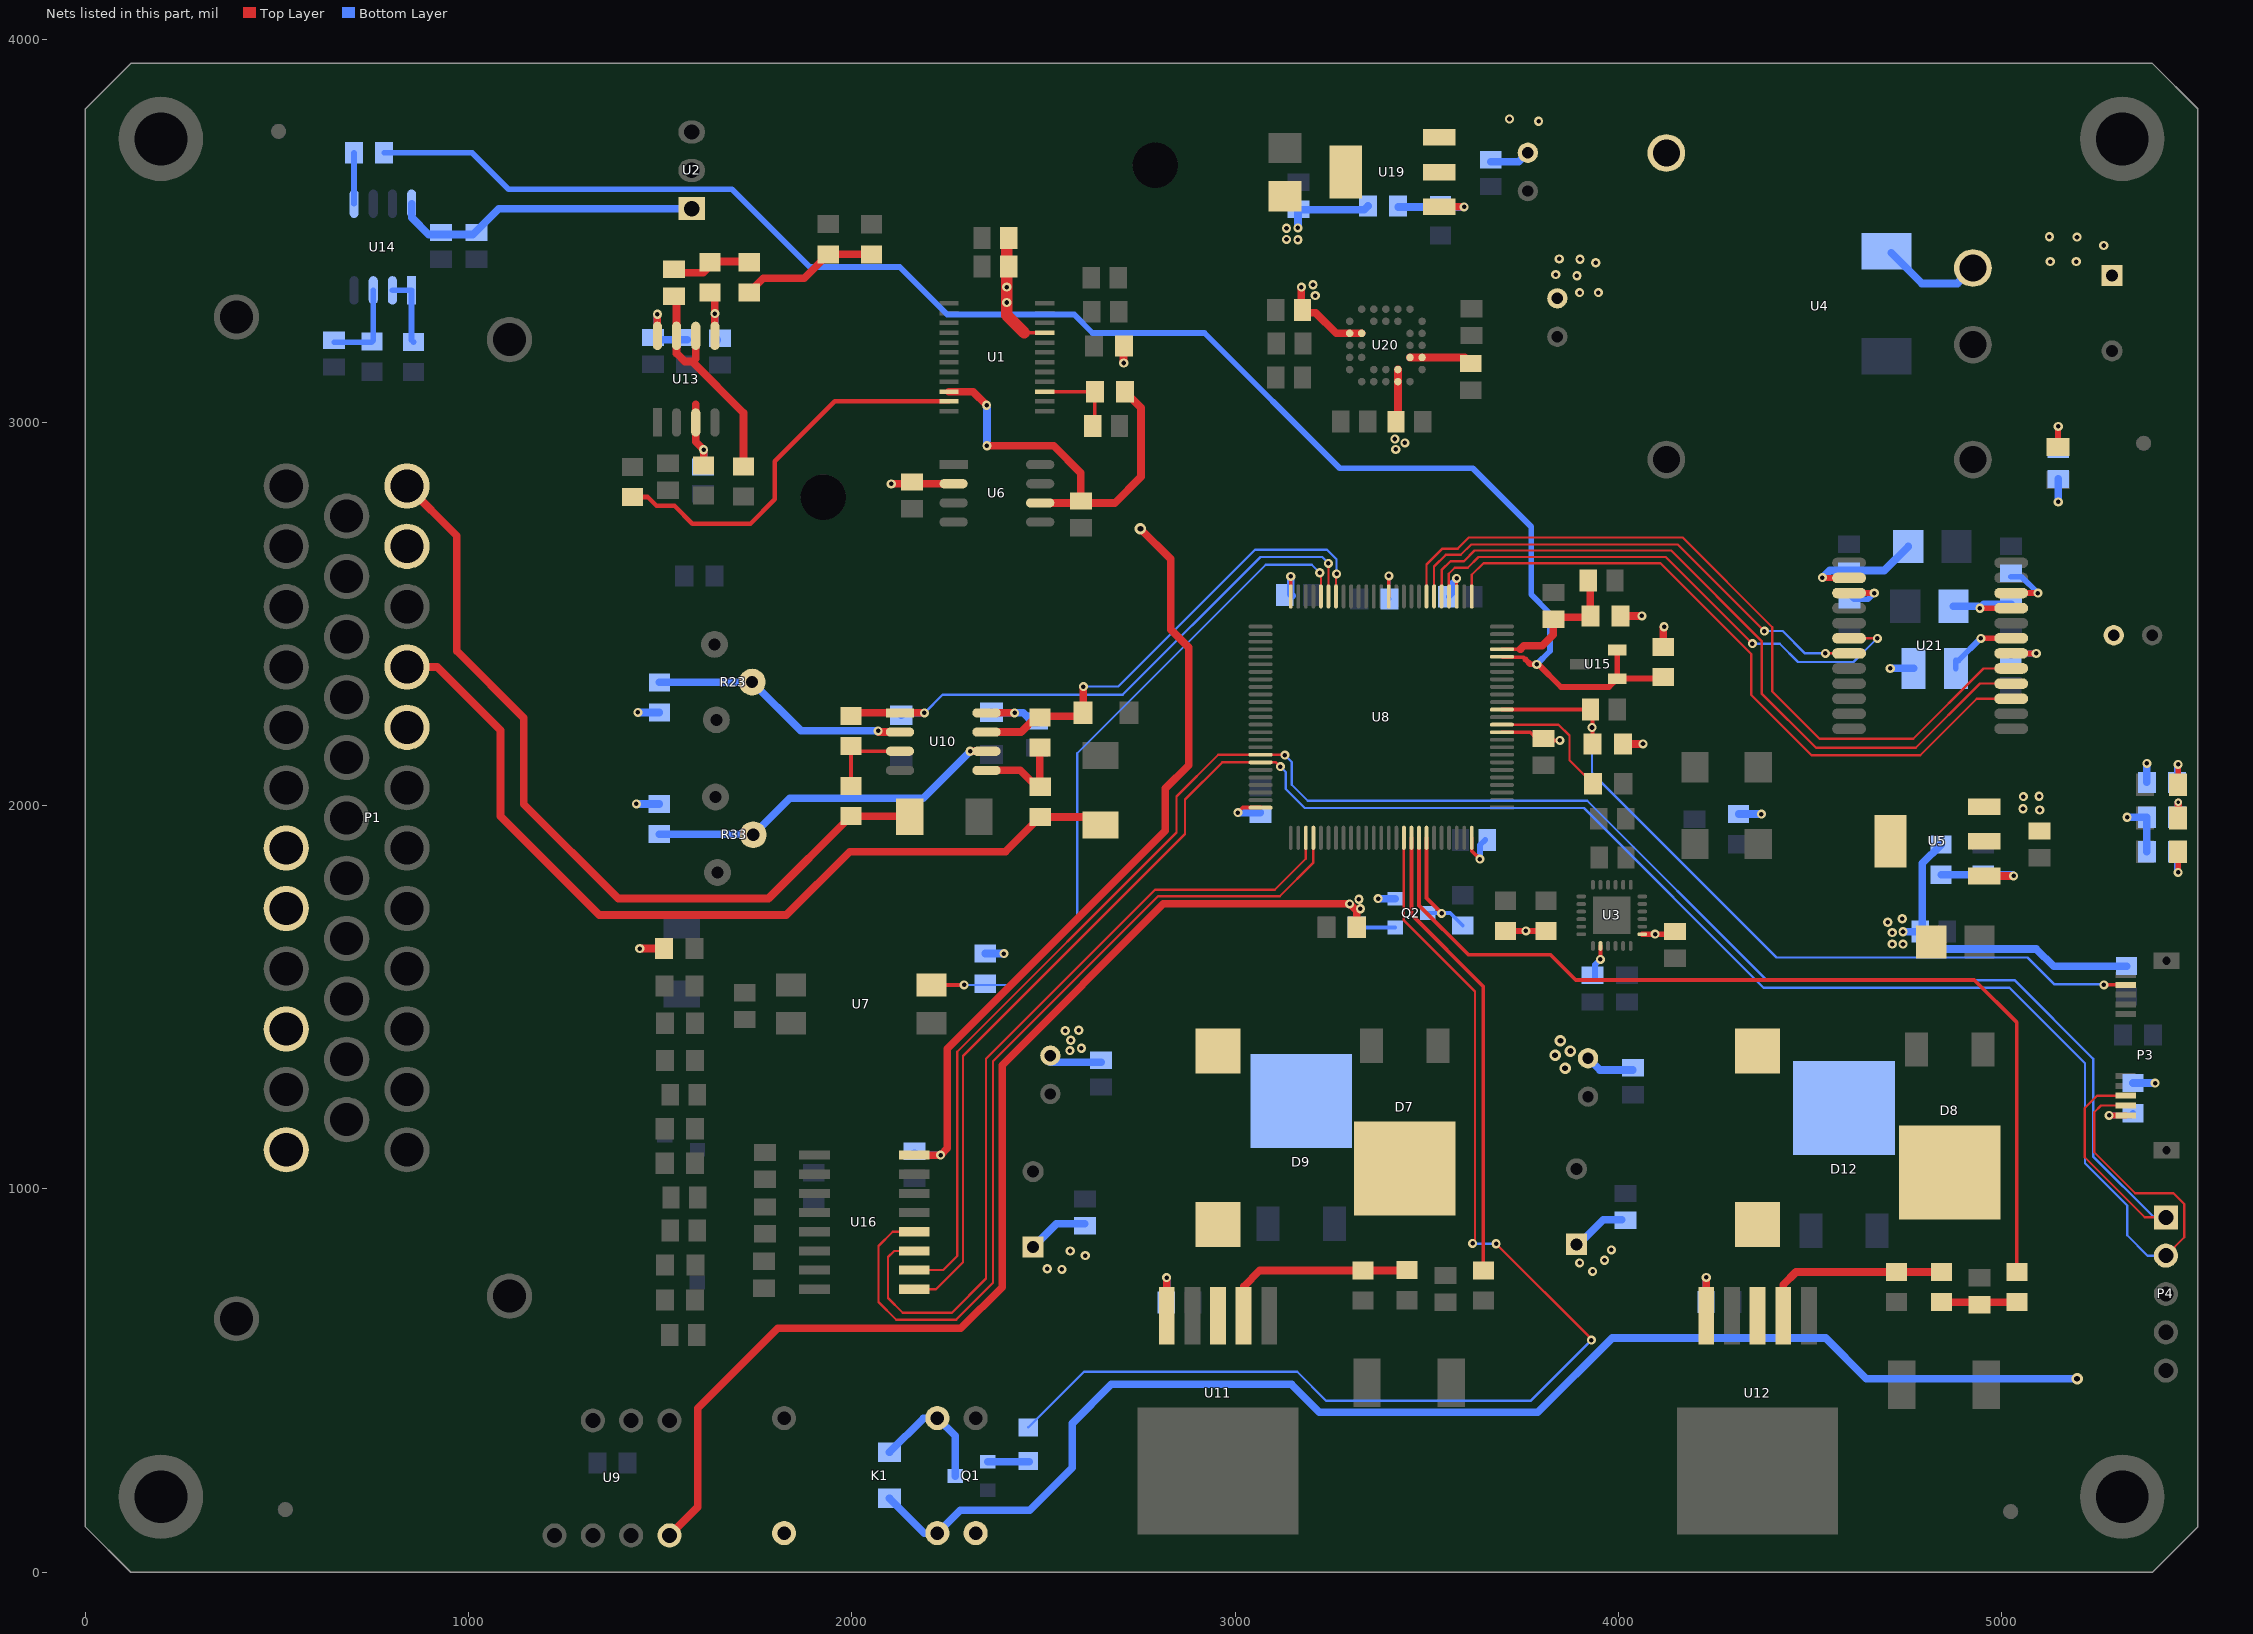
[diagram p0: the nets of this part, all layers, seen from the top]
# Altium PCB MISC82155.PcbDoc (part 4 of 5)
Units mil, origin at the board's own origin, x right, y up, seen from the top; angles counter-clockwise.
Board outline 5511.81 x 3937.01 mil, 4 copper layers (Top Layer, GND, POWER, Bottom Layer); 191 components, 134 nets, 709 pads, 440 vias.

## Via types
v1: diameter 24, hole 12, Top Layer to Bottom Layer, 278 vias
v2: diameter 23.62, hole 11.81, Top Layer to Bottom Layer, 144 vias
v3: diameter 30, hole 15, Top Layer to Bottom Layer, 17 vias
v4: diameter 20, hole 10, Top Layer to Bottom Layer, 1 vias

## Nets (pads, with @x,y where several pads share a name; then routed paths per layer and width w, separated by ;. In a path a pad name is that pad's centre, name@x,y a point inside that pad or via, vN(x,y) a via of type N, cw(c..) or ccw(c..) an arc to the next point about the centre after c; other vN are vias at no path point) (continued)
NetC60_2: C60.2 U20.C1 U20.C2 | length 165.2
  Top Layer w20: U20.C2@3456.4,3169.85 U20.C1@3487.89,3169.85 3599.15,3169.85 C60.2@3615,3154
NetC65_1: C65.1 U21.15 | length 143
  Top Layer w15: U21.15@4602.17,2555.09 v2(4667.91,2555.09)
  Bottom Layer w15: C65.1@4602.66,2551.93 4615.59,2539 4651.83,2539 v2(4667.91,2555.09)
NetC66_1: C66.1 U21.10 | length 157.5
  Top Layer w15: U21.10@5025.4,2555.09 v2(5094.91,2555.09)
  Bottom Layer w15: C66.1@5024.66,2597.88 5052.12,2597.88 v2(5094.91,2555.09)
NetC67_1: C67.1 U21.6 | length 132.9
  Top Layer w15: U21.6@5025.4,2397.61 v2(5090.61,2397.61)
  Bottom Layer w15: C67.1@5025.66,2390.93 5032.33,2397.61 v2(5090.61,2397.61)
NetC69_1: C69.1 R31.2 R37.2 | length 197
  Top Layer w20: R31.2@4843,704.63 R37.2@5040,704.63
NetC71_1: C71.1 R43.1 U13.6 U13.7 | length 601.4
  Top Layer w20: C71.1@1543.41,3331.81 1542.41,3330.81 U13.7@1542.41,3226.34 1542.41,3180.34 1563.41,3159.34 1583,3159.34 1717,3025.34 R43.1@1717,2893.31 ; 1592.41,3166.34 1592.41,3178.34 U13.6@1592.41,3226.34 ; R43.1@1709.41,2885.71 R43.1@1717,2893.31 ; R43.1@1717,2885.37 R43.1@1717,2893.31
NetC71_2: C71.2 R47.2 R48.1 | length 212.4
  Top Layer w20: C71.2@1551.04,3398.5 1543.41,3390.87 1612.5,3390.87 1642,3420.37 1730,3420.37 R47.2@1732,3418.37
NetC72_1: C72.1 R46.2 U13.3 | length 218.8
  Top Layer w20: 1592.41,3047.34 U13.3@1592.41,3000.34 1592.41,2949.59 v2(1613,2929) R46.2@1613,2888.37
  Bottom Layer w20: C72.1@1611,2878.53 1613,2880.53 v2(1613,2929)
NetC73_1: C73.1 R48.2 U13.5 | length 186.7
  Top Layer w20: R48.2@1642,3341.63 1642,3284.41 v2(1642.41,3284) U13.5@1642.41,3226.34
  Bottom Layer w20: v2(1642.41,3284) 1642.41,3222.12 C73.1@1649,3215.53
NetC78_1: C78.1 R61.1 U14.3 | length 234.6
  Bottom Layer w15: C78.1@649,3209.53 746.16,3209.53 751,3214.37 U14.3@751,3345
NetD1_1: D1.1 R5.1 | length 109.2
  Top Layer w15: v2(5461,1826) D1.1@5461,1880
  Bottom Layer w15: R5.1@5458.06,1880 5458.06,1828.94 v2(5461,1826)
NetD2_1: D2.1 R7.1 | length 81.8
  Top Layer w19.68: D2.1@5461,1968 v4(5461,2009) v4@5461,2009.63
  Bottom Layer w19.68: R7.1@5458.06,1970 5461,1972.94 v4(5461,2009)
NetD3_1: D3.1 R10.1 | length 101.2
  Top Layer w15: D3.1@5461,2055 v2(5461,2108)
  Bottom Layer w15: R10.1@5458.06,2061 5458.06,2105.06 v2(5461,2108)
NetD5_1: D5.1 R3.1 | length 112.2
  Top Layer w15: D5.1@5147.41,2936.65 5147.41,2989.41 v2(5148,2990)
  Bottom Layer w15: R3.1@5148,2931.37 v2(5148,2990)
NetD7_2: D7.2 L5.1 U11.3
NetD8_2: D8.2 L6.1 U12.3
NetD13_1: D13.1 K1.5 Q1.3 | length 332.1
  Bottom Layer w20: D13.1@2098,313 2187,402 K1.5@2223,402 2269.5,355.5 Q1.3@2269.5,251
NetL4_2: L4.2 U21.7 | length 189.1
  Top Layer w15: v2(4946.02,2436.98) U21.7@5025.4,2436.98
  Bottom Layer w15: L4.2@4880.78,2358.41 4880.78,2378.78 4887.82,2378.78 v2(4946.02,2436.98)
NetP3_1: P3.1 R60.2 | length 107.4
  Top Layer w15.75: v2(5281,1192.29) P3.1@5324.16,1192.29
  Bottom Layer w15.75: v2(5281,1192.29) 5337.66,1192.29 R60.2@5343,1197.63
NetQ1_1: Q1.1 R50.2 | length 107.7
  Bottom Layer w20: Q1.1@2354.5,288.4 2461.6,288.4 R50.2@2462,288
NetQ2_1: Q2.1 R34.1 | length 95.7
  Bottom Layer w10: R34.1@3322.03,1682.6 Q2.1@3417.65,1682.6
NetQ2_3: Q2.3 R28.2 U8.94 | length 317.5
  Top Layer w9.84: U8.94@3499.52,1916.38 3499.52,1759.48 v2@3539,1720
  Bottom Layer w9.84: Q2.3@3502.65,1720 3561.63,1720 R28.2@3594,1687.63
  other v2: 3539,1719
NetR2_1: R2.1 R47.1 R49.1 | length 360.3
  Top Layer w20: R47.1@1732,3339.63 1768.95,3376.58 1876.02,3376.58 1934.44,3435 R2.1@1938.41,3438.97 2050.66,3438.97 R49.1@2051,3438.63
NetR14_1: R14.1 R16.2 U11.2 | length 520.4
  Top Layer w20: U11.2@3022.34,669.34 3022.34,745.27 3064.44,787.37 R16.2@3334,787.37 3448,787.37 R14.1@3449,788.37
NetR15_2: R15.2 R19.1 U10.3 | length 237.9
  Top Layer w10: R19.1@1997.41,2051.71 R15.2@1997.41,2155.97 2011.04,2142.34 U10.3@2125.41,2142.34
NetR17_1: R17.1 R21.2 U19.1 | length 237.6
  Top Layer w20: U19.1@3532.33,3562.9 v2(3597.9,3562.9)
  Bottom Layer w20: R17.1@3426,3562.63 3597.63,3562.63 v2(3597.9,3562.9)
NetR22_1: R22.1 R23.2 U10.2 | length 680.7
  Top Layer w20: R23.2@1739.2,2322.14 R23.2@1739.83,2322.77 ; v1@2069.41,2192.34 U10.2@2125.41,2192.34
  Bottom Layer w20: R22.1@1497.62,2322.14 1739.2,2322.14 R23.2@1739.83,2322.77 1867.26,2195.34 v1(2068.41,2195.34)
NetR25_2: R25.2 R29.1 U10.5 | length 241.1
  Top Layer w20: U10.5@2351.41,2092.34 2439.66,2092.34 2469.66,2062.34 R29.1@2478.79,2062.34 ; R29.1@2490.41,2050.72 R25.2@2490.41,2151.97
NetR26_2: R26.2 R31.1 U12.2 | length 507.1
  Top Layer w20: U12.2@4430.34,669.34 4430.34,750 4463.71,783.37 R26.2@4726,783.37 R31.1@4843,783.37
NetR32_1: R32.1 R33.2 U10.6 | length 945
  Top Layer w20: v1(2308.41,2142.34) U10.6@2351.41,2142.34
  Bottom Layer w20: R32.1@1497.41,1925.97 1740.99,1925.97 R33.2@1742.62,1924.34 1838.28,2020 2186.07,2020 v1(2308.41,2142.34)
NetR35_1: R35.1 R38.2 U5.1 | length 268
  Top Layer w20: U5.1@4954.45,1816.79 v2(5031.79,1816.79)
  Bottom Layer w20: R35.1@4842.41,1819.97 R38.2@4952.41,1819.97 5028.61,1819.97 v2(5031.79,1816.79)
NetR39_2: R39.2 U1.11 | length 1045.1
  Top Layer w12: R39.2@1427,2805.63 1467.37,2805.63 1490,2783 1537,2783 1583.66,2736.34 1735.34,2736.34 1799,2800 1799,2898.93 1955.25,3055.18 U1.11@2253.41,3055.18
NetR54_1: R54.1 U14.1 U14.2 | length 186.7
  Bottom Layer w15: U14.2@801,3345 U14.1@851,3345 851,3215.37 R54.1@856,3210.37
NetR62_2: R62.2 U14.5 | length 132.6
  Bottom Layer w15: U14.5@701,3571 R62.2@701,3703.63
NRST: C17.2 P3.9 R24.1 U8.14 | length 2067.2
  Top Layer w9.84: U8.14@3696.37,2251.03 3932.56,2251.03 3932.88,2251.34 3932.88,2161.5 R24.1@3933.04,2161.34 ; v2(5267.16,1532.84) P3.9@5324.16,1532.84
  Bottom Layer w6: v1(3931.41,2204.34) 3931.41,2085.59 4413,1604 5068,1604 5138.16,1533.84 5266.16,1533.84 v2(5267.16,1532.84)
PB2_BOOT1: R20.2 U8.37 | length 115
  Top Layer w9.84: U8.37@3401.09,2546.3 v2(3401.09,2599.91)
  Bottom Layer w9.84: v2@3401,2600 v2(3401.09,2599.91) 3401.09,2541.03 R20.2@3402.78,2539.34
PD_IN: R9.2 U7.4 U8.46 | length 1812.4
  Top Layer w6: v2(3220.85,2608) 3223.93,2604.93 U8.46@3223.93,2546.3
  Top Layer w9.84: U7.4@2217.11,1522.71 U7.4@2207.48,1532.34 v2(2293,1532.34)
  Bottom Layer w6: v2(2293,1532.34) 2422.34,1532.34 2588,1698 2588,2137 3080,2629 3199.85,2629 v2(3220.85,2608)
  Bottom Layer w9.84: v2@2291.37,1530.71 v2(2293,1532.34)
REF1: C3.1 R1.1 U1.15 | length 219
  Top Layer w10: U1.15@2503.84,3080.34 R1.1@2634.04,3080.34 ; C3.1@2633.88,2991.34 R1.1@2633.88,3080.18
REF2V5: R18.2 R62.1 U8.21 U15.1 U15.2 | length 4336.2
  Top Layer w10: U8.21@3696.37,2388.82 3697.68,2387.51 3752.24,2387.51 3758.11,2381.64
  Top Layer w15: 3758.11,2381.64 3770.41,2369.34 3791,2369.34 3850.34,2310 3975.61,2310 U15.1@3997.21,2331.6 ; U15.2@3997.21,2406.4 U15.1@3997.21,2331.94 ; R18.2@4124.04,2331.94 U15.1@3997.55,2331.94 ; U15.1@3997.21,2331.6 U15.1@3997.55,2331.94 ; U15.1@3997.21,2331.6 U15.1@3997.21,2331.94 ; U15.1@3997.21,2331.94 U15.1@3997.55,2331.94
  Bottom Layer w15: R62.1@779.37,3704 1009,3704 1104,3609 1687,3609 1890,3406 2125,3406 2249,3282 2580,3282 2628,3234 2920,3234 3273,2881 3620,2881 3773,2728 3773,2551 3822,2502 3822,2404 v1(3787,2369)
REF2V5_1: C13.1 R1.2 U1.10 U6.6 | length 1101.4
  Top Layer w10: U6.6@2491.41,2790.34 U6.6@2491.88,2789.87
  Top Layer w20: U1.10@2253.41,3080.77 2315.97,3080.77 v1(2351.41,3045.34) ; v1(2352.41,2939.34) 2526.41,2939.34 2597.41,2868.34 C13.1@2597.41,2789.87 ; U6.6@2491.88,2789.87 C13.1@2597.41,2789.87 ; R1.2@2712.78,3080.34 2754.41,3038.71 2754.41,2858.34 2685.93,2789.87 C13.1@2597.41,2789.87
  Bottom Layer w20: v1(2352.41,2939.34) v1@2352.41,3044.34
RXD1: P3.2 P4.2 U8.69 U16.9 | length 5629.9
  Top Layer w6: U16.9@2191.41,738.34 U16.9@2162.41,738.34 2219.34,738.34 2290,809 2290,1347 2869,1926 2869,2016 2966.23,2113.23 U8.69@3066.45,2113.23 3106.77,2113.23 v2(3118,2102) ; P3.2@5324.16,1217.88 5259.88,1217.88 5242,1200 5242,1096 5349,989 5449,989 5477,961 5477,874 P4.2@5429,826
  Bottom Layer w6: v2(3118,2102) 3132,2088 3132,2044 3182,1994 3910.18,1994 4379.18,1525 5021,1525 5218,1328 5218,1067 5328,957 5328,879 5381,826 P4.2@5429,826
RXD2: U8.79 U16.12 | length 2305.5
  Top Layer w6: U16.12@2162.41,888.34 2106.41,888.34 2069.41,851.34 2069.41,705.34 2115.75,659 2272,659 2368,755 2368,1333 2799,1764 3116.24,1764 3204.24,1852 U8.79@3204.24,1916.38
SCC_CLK: U8.30 U21.4 | length 1939.2
  Top Layer w6: U8.30@3538.89,2546.3 3538.89,2614.89 3562,2638 3597,2638 3625,2666 4138,2666 4374,2430 4374,2293 4515.79,2151.21 4776.21,2151.21 4943.87,2318.87 U21.4@5025.4,2318.87
SCC_CS: U8.29 U21.18 | length 1409.2
  Top Layer w6: U8.29@3558.57,2546.3 3557.45,2547.43 3557.45,2605.45 3573,2621 3607,2621 3635,2649 4124,2649 v2(4350,2423) ; U21.18@4602.17,2436.98 v2(4675.98,2436.98)
  Bottom Layer w6: v2(4350,2423) 4421,2423 4469,2375 4614,2375 v2(4675.98,2436.98)
SCC_MISO: U8.32 U21.5 | length 2039.3
  Top Layer w6: U8.32@3499.52,2546.3 3499.52,2629.52 3541,2671 3581,2671 3610,2700 4168,2700 4402,2466 4402,2298 4524.97,2175.03 4769.79,2175.03 4953,2358.24 U21.5@5025.4,2358.24 U21.5@5034.66,2358.24
SCC_MOSI: U8.31 U21.19 | length 1371.2
  Top Layer w6: 3519.2,2579.55 U8.31@3519.2,2546.3 3519.2,2624.2 3550,2655 3589,2655 3616,2682 4155,2682 4364,2473 v2(4381,2456) ; v2(4540.61,2397.61) U21.19@4602.17,2397.61 U21.19@4566.86,2397.61
  Bottom Layer w6: v2(4381,2456) 4429,2456 4487.39,2397.61 v2(4540.61,2397.61)
SCC_RST: U8.26 U21.3 | length 1838.6
  Top Layer w6: U8.26@3617.63,2546.3 3617.63,2602.63 3648,2633 4110,2633 4347,2396 4347,2289 4504,2132 4788,2132 4935.5,2279.5 U21.3@5025.4,2279.5 U21.3@4994.75,2279.5
SEAT_PRESS: DW3.2 R15.1 U8.45 U10.1 | length 1581.1
  Top Layer w6: U8.45@3243.61,2546.3 v2(3243.61,2632.61)
  Top Layer w20: R15.1@1987,2242.34 U10.1@2125.41,2242.34 v2(2189.34,2242.34)
  Bottom Layer w6: v2(2189.34,2242.34) 2237,2290 2707,2290 3066,2649 3227.22,2649 v2(3243.61,2632.61)
  Bottom Layer w20: DW3.2@2129,2236 2135.34,2242.34 v2(2189.34,2242.34)
SEAT_SEN: D10.2 P1.1 R19.2 | length 2155.3
  Top Layer w20: P1.1@838.99,2834.48 969,2704.47 969,2404 1144,2229 1144,2004 1390,1758 1782.44,1758 R19.2@1997.41,1972.97 2149.23,1972.97 D10.2@2150.85,1971.34
SO_12V: C18.1 C19.1 C20.1 C33.1 C34.1 C38.1 K1.2 U11.5 U12.5 | length 637.2
  Top Layer w20: U11.5@2821.55,669.34 v2(2821.55,768.55) ; U12.5@4229.55,669.34 v2(4229.55,769.45)
  Bottom Layer w20: C18.1@2473,848.57 2533.9,909.47 C19.1@2608,909.47 ; v2(2821.55,768.55) 2821.55,707.92 C20.1@2825.47,704 ; C33.1@3891,855.57 3896.76,855.57 3961,919.81 C34.1@4009.41,919.81 ; v2(4229.55,769.45) 4229.55,709.92 C38.1@4234.47,705
  other v1: 3933,785 2548,790 2510,792 3899,807 3964,814 2609,826 2570,838 3982,841
SO_PW: R50.1 U8.91 | length 3179
  Top Layer w6: U8.91@3440.46,1916.38 3440.46,1700.54 3626,1515 3626,864 v2(3620,858) ; v2(3681,857) 3929.69,608.31 v2(3929.69,605.69)
  Bottom Layer w6: R50.1@2460,378 2461,378 2606,523 3162,523 3238,447 3771,447 v2(3929.69,605.69) ; v2@3621,857 v2(3681,857)
SOLENIOD_A: C21.1 C31.1 D9.2 L5.2 P1.35 | length 135.3
  Bottom Layer w20: C31.1@2515.41,1332.34 2517.22,1330.53 C21.1@2650,1330.53
  other v1: 2569,1361 2599,1367 2571,1388 2557,1413 2592,1414
SOLENIOD_B: C43.1 C68.1 D12.2 L6.2 P1.33 | length 129.6
  Bottom Layer w20: C68.1@3921,1341 3951.47,1310.53 C43.1@4038,1310.53
  other v3: 3861,1315 3835,1349 3875,1360 3849,1387
STWHEEL_SEN: D11.2 P1.4 R29.2 | length 2326.6
  Top Layer w20: P1.4@838.99,2362.04 917.96,2362.04 1083,2197 1083,1973 1341,1715 1829,1715 1994,1880 2400.67,1880 R29.2@2491.53,1970.86 D11.2@2660.41,1970.86
SUOFA_IN: DW4.2 R25.1 U8.44 U10.7 | length 1249.4
  Top Layer w6: U8.44@3263.3,2546.3 3263.3,2605.3 v2(3264.7,2605.3)
  Top Layer w20: U10.7@2351.41,2192.34 2441.34,2192.34 2479.71,2230.71 R25.1@2490.41,2230.71 ; R25.1@2489.41,2233.34 DW4.2@2598.04,2233.34 ; DW4.2@2603.41,2242.34 v2@2603.41,2311
  Bottom Layer w6: v2(2604,2311) 2695,2311 3052,2668 3240,2668 3264.7,2643.3 v2(3264.7,2605.3)
TXD1: P3.3 P4.1 U8.68 U16.10 | length 5433.6
  Top Layer w6: U16.10@2195.41,788.34 U16.10@2162.41,788.34 2238.34,788.34 2275,825 2275,1358 2847,1930 2847,2024 2955.92,2132.92 U8.68@3066.45,2132.92 3129.08,2132.92 v2(3130,2132) ; P3.3@5324.16,1243.47 5249.47,1243.47 5217,1211 5217,1083 5374,926 P4.1@5429,926
  Bottom Layer w6: v2(3130,2132) 3148,2114 3148,2054.57 3189.57,2013 3919,2013 4387,1545 5034,1545 5239,1340 5239,1085 5398,926 P4.1@5429,926
TXD2: U8.78 U16.11 | length 2169.1
  Top Layer w6: U16.11@2162.41,838.34 2110.41,838.34 2094.41,822.34 2094.41,715.34 2132.75,677 2261,677 2350,766 2350,1340 2791,1781 3103.56,1781 3184.56,1862 U8.78@3184.56,1916.38
VALVE_PWM1: R30.1 U8.92 | length 1223.8
  Top Layer w9.84: 3460.15,1876.08 3460.15,1884 ; U8.92@3460.15,1916.38 3460.15,1884 ; 3647.41,874.97 3647.41,884 ; R30.1@3648,787.37 3647.41,787.96 3647.41,884 ; 3460.15,1884 3460.15,1716 3647.41,1528.74 3647.41,884
VALVE_PWM2: R37.1 U8.93 | length 2513.9
  Top Layer w9.84: U8.93@3479.83,1916.38 3479.83,1740 3608.83,1611 3823,1611 3889,1545 4929,1545 5040,1434 R37.1@5040,783.37
VCCA: C36.2 C37.2 L3.2 U8.22 | length 390.4
  Top Layer w10: U8.22@3696.37,2408.51 3744.57,2408.51 3746.41,2410.34
  Top Layer w20: 3744.57,2408.51 3753.25,2417.19 3801.19,2417.19 3830.41,2446.41 C37.2@3830.41,2491.81 ; C37.2@3827.88,2491.81 C37.2@3830.41,2491.81 ; C36.2@3926.88,2587.34 3926.88,2495.5 L3.2@3927.04,2495.34 3923.51,2491.81 C37.2@3830.41,2491.81
VDD_3.3: C8.1 C12.2 C14.1 C15.1 C23.1 C24.1 C25.1 C26.1 C27.1 C41.2 C42.2 C61.1 C62.1 C63.1 C64.1 L2.2 L3.1 L4.1 Q2.2 R9.1 R24.2 R35.2 R41.2 R42.2 R45.1 R55.2 U1.21 U3.8 U3.13 U5.2 U8.11 U8.28 U8.50 U8.75 U8.100 U9.4 U21.9 U21.14 | length 6041.2
  Top Layer w8: U8.28@3578.26,2546.3 v2(3578.26,2593.34)
  Top Layer w10: 2449.43,3234.32 U1.21@2503.41,3234.32 ; v2(3007,1982) 3020.12,1995.12 U8.75@3066.45,1995.12 ; U8.50@3145.19,2546.3 v2(3145.19,2598.34) v2@3145.19,2603.03 ; 3617.63,1881.34 3617.63,1882.37 ; U8.100@3617.63,1916.38 3617.63,1882.37 ; v2(3639,1861) 3617.63,1882.37 ; U8.11@3696.37,2191.97 3770.3,2191.97 C23.1@3785.41,2176.87 ; C23.1@3804.41,2169.87 3846.93,2169.87 v2(3847.41,2170.34) ; v2(3953,1599) 3953.47,1599.47 U3.8@3953.47,1634.28 ; C41.2@4147,1666.47 C41.2@4147.21,1666.26 ; v1(4532.66,2595.41) v1@4533.61,2594.46
  Top Layer w15: R42.2@3705.32,1673.44 v2(3759,1673.44) R41.2@3811.32,1673.44 ; U3.13@4062.72,1664.79 v2@4099,1664.79 ; v2(4096.21,1664.79) v2@4099,1664.79 ; C41.2@4148,1666.53 4146.26,1664.79 v2@4099,1664.79 ; v1@4533.61,2594.46 U21.14@4602.17,2594.46 ; v1@4943.66,2515.72 U21.9@5025.4,2515.72
  Top Layer w20: U9.4@1524,96 1598,170 1598,428 1806.5,636.5 2284.5,636.5 2392,744 2392,1323 2813,1744 v2(3299,1744) 3317.37,1725.63 R55.2@3317.37,1683 ; L3.1@4005.78,2495.34 v2(4061.41,2495.34) ; R24.2@4011.78,2161.34 v2(4064.41,2161.34)
  Top Layer w30: C14.1@2403.93,3481.34 2403.93,3407.34 v1(2403.93,3353.34) 2403.93,3279.81 2449.43,3234.32
  Bottom Layer w15: C24.1@3557.88,2545.34 3566,2553.46 3566,2581.08 v2(3578.26,2593.34) ; v2(3639,1861) 3639,1897.47 C26.1@3652.53,1911 ; C42.2@3939,1549.53 3939,1585 v2(3953,1599)
  Bottom Layer w20: R9.1@2348,1614.37 v2(2396.37,1614.37) ; v2(3007,1982) 3007.47,1982.47 C25.1@3066,1982.47 ; v2(3145.19,2598.34) 3145.19,2552.03 C27.1@3148.88,2548.34 ; v2(3373.4,1757.4) Q2.2@3417.65,1757.4 ; L2.2@4314,1978.37 v2(4373.63,1978.37) ; v1(4532.66,2595.41) 4532.89,2595.41 4551.36,2613.88 4602.66,2613.88 4694.14,2613.88 C61.1@4756.67,2676.41 ; v2(4709.59,2358.41) L4.1@4770.54,2358.41 ; v1(4743,1671) 4792.47,1671 4793.47,1672 4793.47,1747 ; C12.2@4793.47,1659.22 4826.69,1626 5091,1626 5136,1581 5325.63,1581 R45.1@5326,1581.37 ; 4793.47,1820.78 4793.47,1747 ; R35.2@4842.41,1898.71 4793.47,1849.78 4793.47,1747 ; C62.1@4874.65,2520.41 4938.66,2520.41 v1(4943.66,2515.41) 4954.19,2525.93 C64.1@5024.66,2525.93
  other v1: 4715,1639 4743,1639 4715,1669 4703,1696 4741,1705 3327,1731 3323,1756 2403.93,3313.34
VDD_5V: C10.1 C11.2 C35.1 C46.1 C70.2 C74.1 C75.1 C76.1 C77.1 D13.2 K1.4 L1.1 R3.2 R5.2 R7.2 R10.2 R18.1 R60.1 U2.1 U4.3 U5.3 U6.2 U13.8 U14.8 U16.16 | length 7204.7
  Top Layer w20: U13.8@1492.41,3226.34 v2(1492.41,3282.59) ; v1(2102.88,2839.87) C11.2@2162.41,2839.87 ; U16.16@2162.41,1088.34 v2(2231.41,1088.34) 2249,1105.93 2249,1366 2818,1935 2818,2045 2879,2106 2879,2413 2832,2460 2832,2644 v3(2753,2723) ; C11.2@2162.88,2840.34 U6.2@2265.41,2840.34 ; v1@2708.78,3155.97 L1.1@2708.78,3209.34 ; R18.1@4117.41,2414.71 4117.41,2465.34 v1(4119.41,2467.34)
  Bottom Layer w20: U14.8@851,3571 851,3535 895.47,3490.53 928,3490.53 1011,3490.53 1078.47,3558 U2.1@1582,3558 ; v2(1492.41,3282.59) 1492.41,3215.87 C74.1@1570.41,3215.87 ; D13.2@2098,193 2189,102 K1.4@2223,102 2283,162 2464,162 2575,273 2575,388 2677,490 3147,490 3220,417 3790,417 3984,611 4541,611 4647,505 v3(5197,505) ; C46.1@2163.41,1092.87 2167.93,1088.34 v2(2231.41,1088.34) ; v2(5148,2793) R3.2@5148,2852.63 ; v2(5328,1970) R7.2@5379.32,1970 R5.2@5379.32,1880 ; R60.1@5343,1276.37 v2(5400.63,1276.37) ; R10.2@5379.32,2061 v2(5379.32,2110.68)
  other v1: 5100,1989 5056,1992 5057,2024 5098,2025 2709.41,3155.34 3899,3339 3948,3339 3892,3383 3837,3386 3941,3417 3900,3426 3846,3427
VDD_6V: C6.1 C9.2 C39.2 C44.2 R17.2 U19.2 U20.A3 U20.B3 U20.E6 U20.E7 | length 612.1
  Top Layer w20: v1(3172.93,3353.34) 3172.93,3292.34 3178.36,3286.91 3209.83,3286.91 3263.91,3232.84 U20.E7@3298.92,3232.84 U20.E6@3330.41,3232.84 ; C44.2@3424.9,2999.36 U20.A3@3424.9,3106.85 U20.B3@3424.9,3138.35
  Bottom Layer w20: v1(3164,3508) 3164,3548.47 3170.53,3555 3336.63,3555 R17.2@3346.63,3565
  other v1: 3419,2930 3443,2947 3417,2957 3209.41,3331.34 3203.41,3359.34 3164,3477 3134,3478 3134,3507
VDD_12V: C1.1 C7.2 C29.1 C30.1 C40.1 D6.2 K1.1 P1.2 P1.5 P1.30 P1.31 R11.2 R22.2 R32.2 U4.1 U10.8 U19.3 | length 753.3
  Top Layer w20: v1(1446.41,1627.34) R11.2@1510.04,1627.34 ; U10.8@2351.41,2242.34 v2(2424.66,2242.34)
  Bottom Layer w20: v2(1437.71,2004.71) R32.2@1497.41,2004.71 ; v2(1441.4,2243.4) R22.2@1497.62,2243.4 ; C30.1@2364,2244 2365.66,2242.34 v2(2424.66,2242.34) 2446.66,2242.34 2473.47,2215.53 C29.1@2483,2215.53 ; C7.2@3667,3680.53 3740.53,3680.53 C1.1@3764,3704 ; D6.2@4712.19,3442.81 4792,3363 4885.07,3363 U4.1@4925.41,3403.34
  other v1: 5127,3420 5195,3420 5267,3462 5197,3484 5125,3485 3792,3786 3716,3792
XTAL1: R36.1 U8.12 | length 339.3
  Top Layer w6: U8.12@3696.37,2211.66 3844.09,2211.66 3872.41,2183.34 3872.41,2118.97 R36.1@3934.04,2057.34
pads on no net: K1.3 K1.6 P1.36 P1.37 P1.38 P1.39 P3.0 P3.4 P3.10 R23.3 R33.3 U1.1 U1.2 U1.5 U1.6 U1.7 U1.8 U2/.1 U2/.2 U3.2 U3.3 U3.4 U3.5 U3.6 U3.7 U3.14 U3.15 U3.16 U3.17 U3.19 U3.21 U3.22 U4.6 U6.1 U6.3 U6.5 U6.7 U6.8 U8.1 U8.2 U8.3 U8.4 U8.5 U8.6 U8.7 U8.8 U8.9 U8.13 U8.15 U8.16 U8.17 U8.18 U8.38 U8.39 U8.40 U8.41 U8.42 U8.43 U8.47 U8.56 U8.57 U8.58 U8.59 U8.60 U8.61 U8.62 U8.63 U8.64 U8.65 U8.66 U8.67 U8.73 U8.77 U8.80 U8.89 U8.90 U8.97 U9.5 U11.0 U12.0 U20.D1 U20.D2 U20.F3 U20.F4 U20.F5 U20.G3 U20.G4 U20.G5 U21.2 U21.11 U21.20 U21.21 U21.22 U21.23 Y1.1

## Polygon pours and split planes (outlines as drawn)
VDD_5V on Top Layer "Top Layer-No Net" (solid, remove dead copper, pour order 1000): 4908,2007 4908,1977 4908,1976 4911,1973 4913,1971 4924,1971 5040,1971 5050,1961 5058,1953 5058,1937 5058,1919 5065,1912 5072,1905 5079,1905 5128,1905 5132,1909 5133,1910 5133,1930 5133,2015 5114,2034 5109,2039 5090,2039 4925,2039 4915,2029 4908,2022 4908,2007
VDD_3.3 on Top Layer "Top Layer-No Net" (solid, remove dead copper, pour order 32): 4646,1903 4646,1876 4609,1839 4585,1815 4585,1746 4585,1703 4679,1609 4698,1590 4783,1590 4855,1590 4862,1597 4865,1600 4865,1636 4865,1826 4889,1850 4921,1882 4961,1882 5027,1882 5030,1885 5032,1887 5032,1893 5032,1932 5027,1937 5026,1938 5015,1938 4858,1938 4806,1990 4791,2005 4757,2005 4691,2005 4671,1985 4646,1960 4646,1903
VDD_5V on Top Layer "Top Layer-No Net" (solid, remove dead copper, pour order 30): 3806,3383 3806,3314 3813,3307 3825,3295 3844,3295 3989,3295 4046,3352 4142,3448 4142,3520 4142,3553 4186,3597 4189,3600 4189,3688 4189,3733 4172,3750 4161,3761 4120,3761 4065,3761 4051,3747 4043,3739 4043,3702 4043,3593 3992,3542 3909,3459 3864,3459 3844,3459 3824,3439 3806,3421 3806,3383
VDD_6V on Top Layer "Top Layer-No Net" (solid, remove dead copper, pour order 28): 3067,3574 3067,3460 3081,3446 3087,3440 3138,3440 3192,3440 3205,3440 3341,3576 3383,3618 3478,3618 3574,3618 3582,3626 3584,3628 3584,3640 3584,3677 3575,3686 3574,3687 3556,3687 3392,3687 3353,3726 3340,3739 3308,3739 3261,3739 3228,3706 3220,3698 3220,3686 3220,3661 3213,3654 3191,3632 3175,3632 3084,3632 3076,3624 3067,3615 3067,3574
VDD_6V on Top Layer "Top Layer-No Net" (solid, remove dead copper, pour order 26): 3150,3326 3150,3265 3152,3263 3154,3261 3155,3261 3221.37,3261 3228.56,3268.19 3231,3270.63 3231,3278 3231,3292 3227,3296 3225,3298 3225,3320 3225,3364 3219,3370 3216,3373 3206,3373 3172,3373 3160,3361 3150,3351 3150,3326
VDD_6V on Top Layer "Top Layer-No Net" (solid, remove dead copper, pour order 24): 3400,3015 3400,2928 3409,2919 3415,2913 3420,2913 3445,2913 3457,2925 3466,2934 3466,2945 3466,2947 3455,2958 3449,2964 3449,2978 3449,3029 3433,3045 3430,3048 3424.9,3048 3419,3048 3414,3043 3400,3029 3400,3015
SOLENIOD_B on Top Layer "Top Layer-No Net" (solid, remove dead copper, pour order 22): 3817,1375.69 3817,1321.51 3830.85,1306.73 3847.47,1289 3961.03,1289 4424.53,1289 4428.23,1292.94 4431,1295.9 4431,1322.49 4431,1414.1 4426.38,1419.03 4424.53,1421 4403.3,1421 3847.47,1421 3833.62,1406.22 3817,1388.49 3817,1375.69
SOLENIOD_A on Top Layer "Top Layer-No Net" (solid, remove dead copper, pour order 20): 2477,1347 2477,1316 2477,1313 2488,1302 2495,1295 2913,1295 3020,1295 3029,1304 3035,1310 3035,1334 3035,1430 3028,1437 3011,1454 2976,1454 2574,1454 2511,1391 2477,1357 2477,1347
GND_SA on Top Layer "Top Layer-No Net" (solid, remove dead copper, pour order 18): 3287,699 3287,433 3292,428 3295,425 3311,425 3385,425 3388,428 3396,436 3396,584 3396,666 3388,674 3374,688 3374,710 3374,728 3369,733 3367,735 3301,735 3300,735 3293,728 3287,722 3287,699